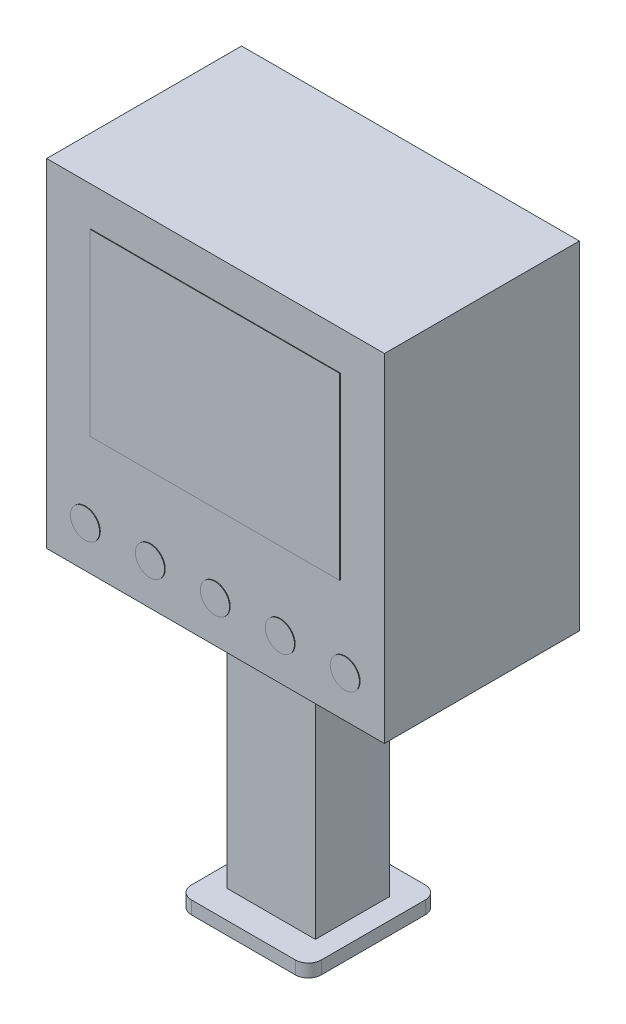
SolidWorks part; units mm, degrees
material "Q235"
ref_plane "Front Plane" through (0, 0, 0) normal (0, 0, 1) x (1, 0, 0)
ref_plane "Top Plane" through (0, 0, 0) normal (0, 1, 0) x (1, 0, 0)
ref_plane "Right Plane" through (0, 0, 0) normal (1, 0, 0) x (0, 0, -1)
sketch "Sketch1" plane through (0, 0, 0) normal (0, 0, 1) x (1, 0, 0)
  line L1 (-130, 130) -> (130, 130)
  line L2 (-130, 130) -> (-130, -130)
  line L3 (-130, -130) -> (130, -130)
  line L4 (130, 130) -> (130, -130)
  line L5 (-130, 130) -> (130, -130) construction
  line L6 (-130, -130) -> (130, 130) construction
  point P0 (0, 0)
  dimension "D1" = 260
  dimension "D2" = 260
extrude "Boss-Extrude1" add sketch "Sketch1" along normal blind 150
sketch "Sketch2" plane through (0, 0, 150) normal (0, 0, 1) x (1, 0, 0)
  line L0 (0, 130) -> (0, -130) construction
  line L1 (-96, 100) -> (96, 100)
  line L2 (-96, 100) -> (-96, -38)
  line L3 (-96, -38) -> (96, -38)
  line L4 (96, 100) -> (96, -38)
  line L5 (130, 130) -> (-130, 130) construction
  line L6 (-130, 130) -> (-130, -130) construction
  line L7 (-130, -130) -> (130, -130) construction
  circle A0 centre (-100, -98) radius 11.25
  circle A1 centre (-50, -98) radius 11.25
  circle A2 centre (0, -98) radius 11.25 construction
  circle A3 centre (50, -98) radius 11.25
  circle A4 centre (100, -98) radius 11.25
  circle A5 centre (0, -98) radius 11.25
  point P9 (0, 100)
  point P23 (0, -98)
  dimension "D4" = 30
  dimension "D7" = 22.5
  dimension "D1" = 192
  dimension "D2" = 138
  dimension "D3" = 30
  dimension "D5" = 50
  dimension "D6" = 50
  dimension "D8" = 32
extrude "Boss-Extrude2" add sketch "Sketch2" along normal blind 0.5
sketch "Sketch3" plane through (0, -130, 0) normal (0, -1, 0) x (1, 0, 0)
  line L1 (-34.0367, 107.1902) -> (34.0367, 107.1902)
  line L2 (-34.0367, 107.1902) -> (-34.0367, 49.9691)
  line L3 (-34.0367, 49.9691) -> (34.0367, 49.9691)
  line L4 (34.0367, 107.1902) -> (34.0367, 49.9691)
  line L5 (-34.0367, 107.1902) -> (34.0367, 49.9691) construction
  line L6 (-34.0367, 49.9691) -> (34.0367, 107.1902) construction
  point P0 (0, 78.5797)
extrude "Boss-Extrude3" add sketch "Sketch3" along normal blind 200
sketch "Sketch4" plane through (0, -330, 0) normal (0, -1, 0) x (1, 0, 0)
  line L0 (0, 107.1902) -> (0, 49.9691) construction
  line L1 (34.0367, 107.1902) -> (-34.0367, 107.1902) construction
  line L2 (-34.0367, 49.9691) -> (34.0367, 49.9691) construction
  line L4 (-50, 128.5797) -> (50, 128.5797)
  line L5 (-50, 128.5797) -> (-50, 28.5797)
  line L6 (-50, 28.5797) -> (50, 28.5797)
  line L7 (50, 128.5797) -> (50, 28.5797)
  line L8 (-50, 128.5797) -> (50, 28.5797) construction
  line L9 (-50, 28.5797) -> (50, 128.5797) construction
  point P6 (0, 78.5797)
  dimension "D1" = 100
  dimension "D2" = 100
extrude "Boss-Extrude4" add sketch "Sketch4" along normal blind 10
fillet "Fillet1" radius 10 4 edges at (50, -335, 28.5797) (-50, -335, 28.5797) (50, -335, 128.5797) (-50, -335, 128.5797)
